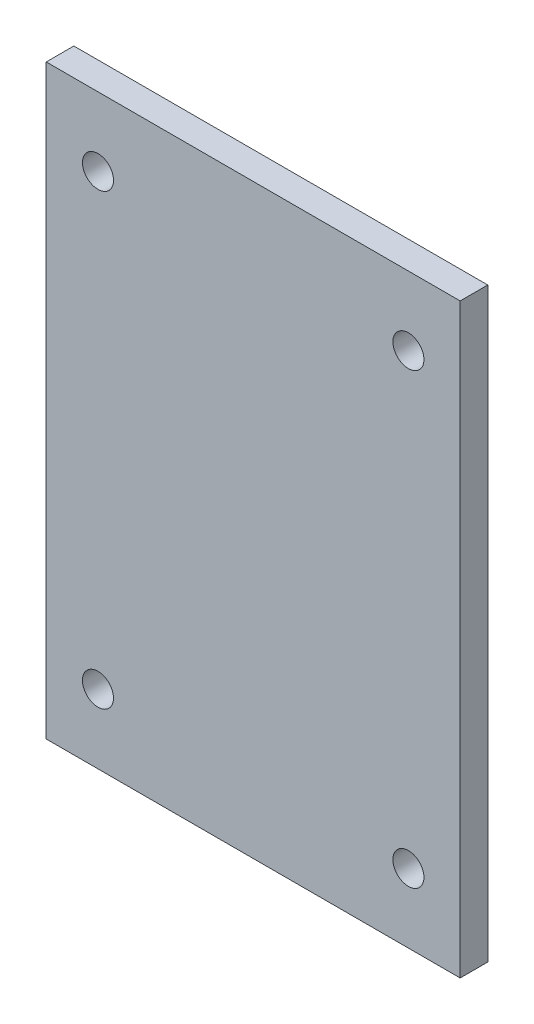
SolidWorks part; units mm, degrees
material "Q235B"
ref_plane "Front Plane" through (0, 0, 0) normal (0, 0, 1) x (1, 0, 0)
ref_plane "Top Plane" through (0, 0, 0) normal (0, 1, 0) x (1, 0, 0)
ref_plane "Right Plane" through (0, 0, 0) normal (1, 0, 0) x (0, 0, -1)
other "Configuration Table"
sketch "Sketch2" plane through (0, 0, 0) normal (0, 0, 1) x (1, 0, 0)
  line L1 (-120, -170) -> (120, -170)
  line L2 (-120, -170) -> (-120, 170)
  line L3 (-120, 170) -> (120, 170)
  line L4 (120, -170) -> (120, 170)
  line L5 (-120, -170) -> (120, 170) construction
  line L6 (-120, 170) -> (120, -170) construction
  circle A0 centre (-90, 130) radius 9
  circle A1 centre (90, 130) radius 9
  circle A2 centre (90, -130) radius 9
  circle A3 centre (-90, -130) radius 9
  point P0 (0, 0)
  dimension "D10" = 18
  dimension "D1" = 240
  dimension "D2" = 340
  dimension "D3" = 180
  dimension "D4" = 130
  dimension "D5" = 130
  dimension "D6" = 130
  dimension "D7" = 90
  dimension "D8" = 90
  dimension "D9" = 90
extrude "Boss-Extrude1" add sketch "Sketch2" along normal blind 16
